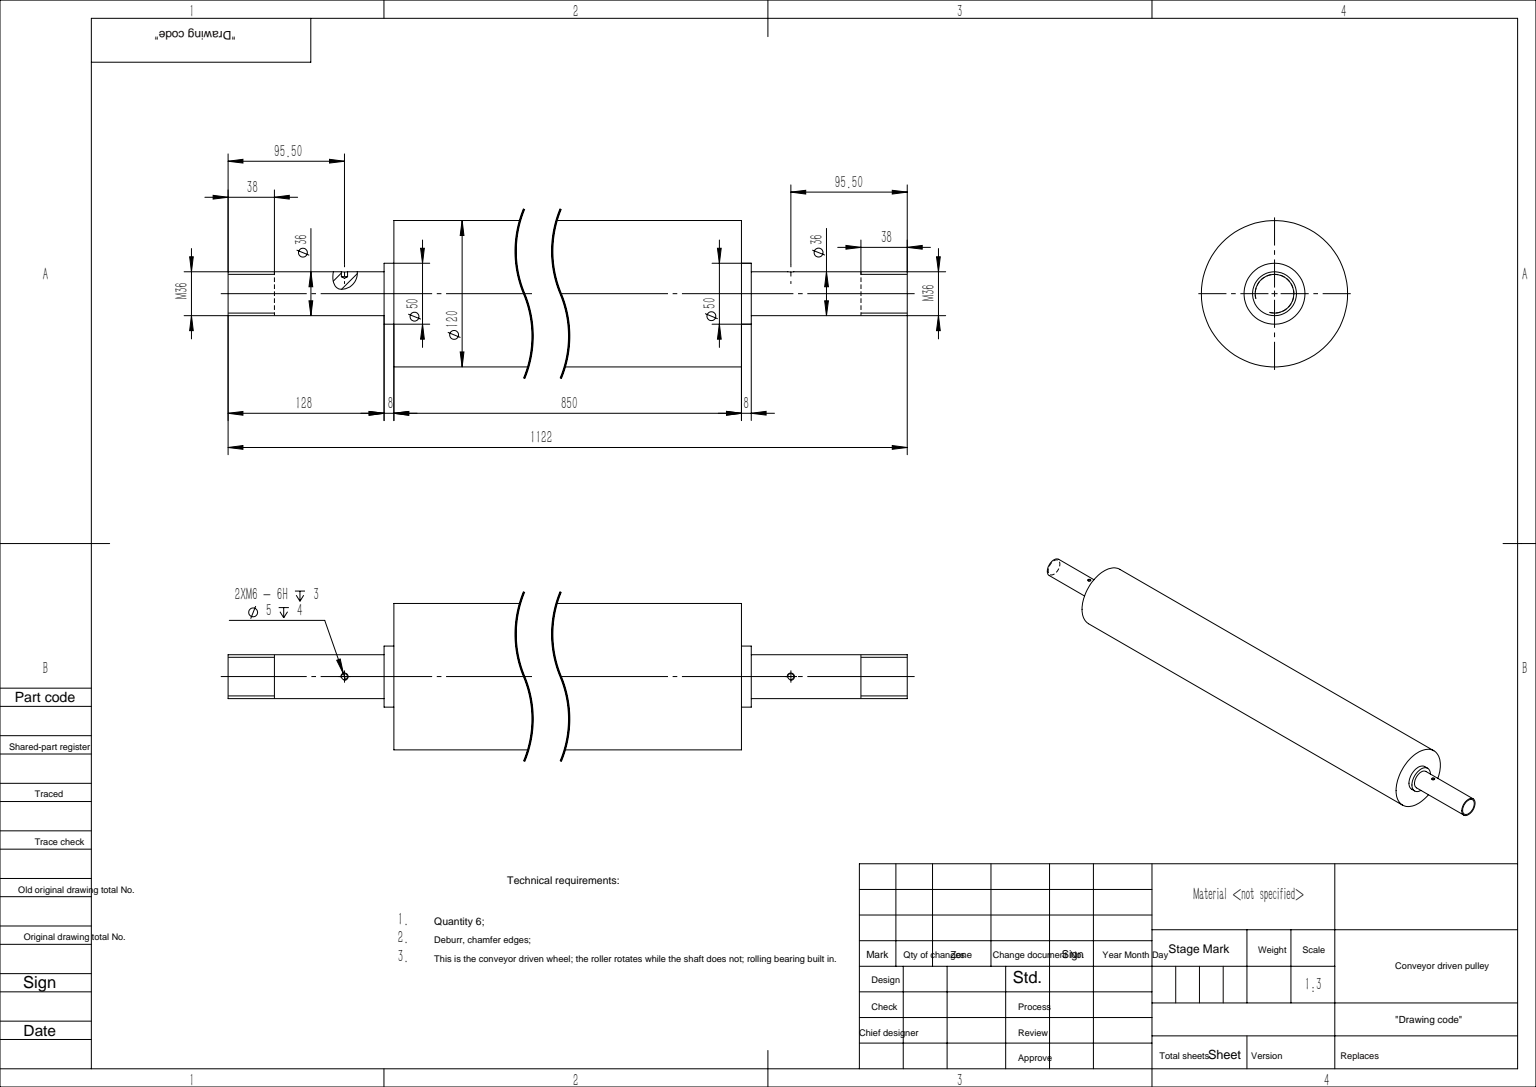
SolidWorks part; units mm, degrees
ref_plane "前视基准面" through (0, 0, 0) normal (0, 0, 1) x (1, 0, 0)
ref_plane "上视基准面" through (0, 0, 0) normal (0, 1, 0) x (1, 0, 0)
ref_plane "右视基准面" through (0, 0, 0) normal (1, 0, 0) x (0, 0, -1)
sketch "草图1" plane through (0, 0, 0) normal (0, 0, 1) x (1, 0, 0)
  line L0 (0, 0) -> (934.2627, 0) construction
  line L1 (0, 0) -> (0, 371.779) construction
  line L2 (-425, 60) -> (425, 60)
  line L3 (425, 60) -> (425, 25)
  line L4 (433, 18) -> (561, 18)
  line L5 (561, 18) -> (561, 0)
  line L6 (-561, 18) -> (-561, 0)
  line L7 (-433, 25) -> (-433, 18)
  line L8 (-433, 18) -> (-561, 18)
  line L9 (-561, 0) -> (561, 0)
  line L10 (425, 25) -> (433, 25)
  line L11 (433, 25) -> (433, 18)
  line L12 (-425, 25) -> (-433, 25)
  line L13 (-425, 60) -> (-425, 25)
  point P13 (0, 60)
  dimension "D1" = 425
  dimension "D2" = 60
  dimension "D3" = 128
  dimension "D4" = 18
  dimension "D5" = 8
  dimension "D6" = 25
revolve "旋转1" add sketch "草图1" angle 360 about L0
cosmetic thread "装饰螺纹线1" parameters "D1"=38, "D2"=31.67
cosmetic thread "装饰螺纹线2" parameters "D1"=38, "D2"=31.67
ref_plane "基准面1" through (0, 0, 18) normal (0, 0, 1) x (1, 0, 0)
hole_wizard "M6 螺纹孔1" positions "3D草图1" profile "草图2" tap size "M6" standard "GB"
sketch3d "3D草图1"
  point P0 (465.5, 18, 0)
  dimension "D1" = 32.5
  dimension "D2" = 18
sketch "草图2" plane through (465.5, 18, 0) normal (1, 0, 0) x (0, 0, 1)
  line L0 (0, 0) -> (0, 5.4434)
  line L1 (0, 5.4434) -> (2.5, 4)
  line L2 (2.5, 4) -> (2.5, 0)
  line L5 (2.5, 0) -> (0, 0)
  line L10 (0, 5.4434) -> (-2.5, 4) construction
  line L11 (0, -6.35) -> (0, 107.95) construction
  dimension "螺纹孔钻头直径" = 5
  dimension "螺纹孔钻头深度" = 4
  dimension "导头角度" = 120
cosmetic thread "孔螺蚊线1" parameters "D1"=3, "D2"=6
mirror "镜向1" about plane through (0, 0, 0) normal (1, 0, 0) of "M6 螺纹孔1"
